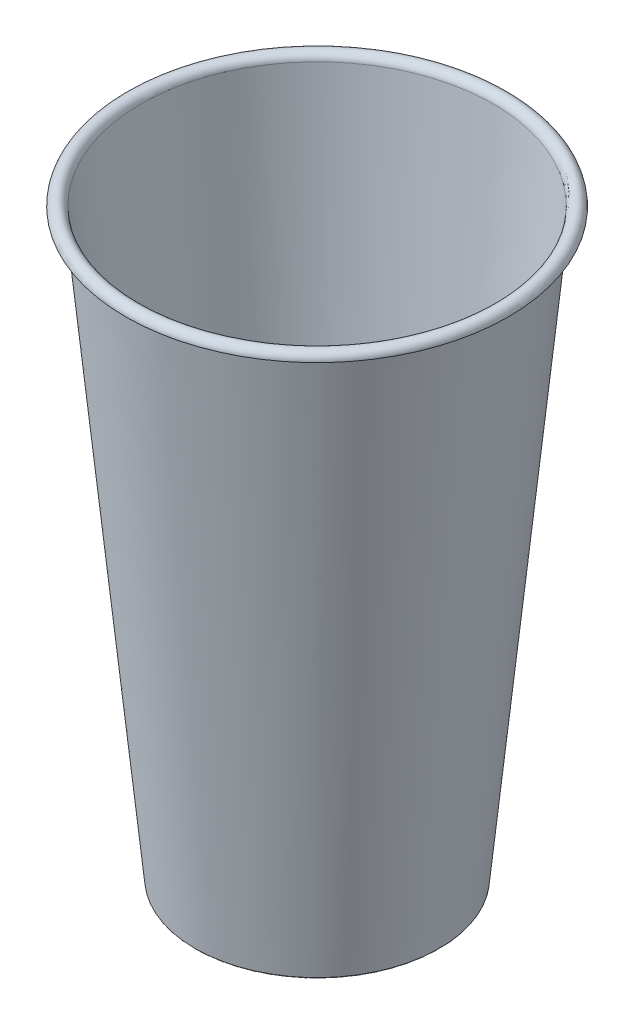
SolidWorks part; units mm, degrees
ref_plane "前视基准面" through (0, 0, 0) normal (0, 0, 1) x (1, 0, 0)
ref_plane "上视基准面" through (0, 0, 0) normal (0, 1, 0) x (1, 0, 0)
ref_plane "右视基准面" through (0, 0, 0) normal (1, 0, 0) x (0, 0, -1)
sketch "草图1" plane through (0, 0, 0) normal (0, 0, 1) x (1, 0, 0)
  line L0 (0, 0) -> (28.15, 0)
  line L1 (27.775, -3.8406) -> (28.0914, -0.6)
  line L2 (0, -0.6) -> (28.0914, -0.6)
  line L3 (28.374, -3.8794) -> (41.5972, 131.5417)
  line L4 (0, 0) -> (0, -0.6)
  line L5 (28.6943, -0.6) -> (41.5972, 131.5417) construction
  line L6 (27.974, -4.06) -> (28.175, -4.06)
  line L7 (28.15, 0) -> (41, 131.6) construction
  line L8 (0, -4.06) -> (28.6943, -4.06) construction
  line L9 (28.15, 0) -> (41, 131.6)
  line L10 (43.8917, 131.4299) -> (44.4917, 131.4299)
  line L11 (0, -0.6) -> (28.6943, -0.6) construction
  arc A0 (44.4917, 131.4299) -> (41, 131.6) centre (42.7417, 131.4299) ccw
  arc A1 (27.974, -4.06) -> (27.775, -3.8406) centre (27.974, -3.86) cw
  arc A2 (28.374, -3.8794) -> (28.175, -4.06) centre (28.175, -3.86) cw
  arc A3 (43.8917, 131.4299) -> (41.5972, 131.5417) centre (42.7417, 131.4299) ccw
  arc A5 (41.4992, 130.1976) -> (41, 131.6) centre (42.7417, 131.4299) ccw construction
  arc A6 (41.9252, 130.6201) -> (41.5972, 131.5417) centre (42.7417, 131.4299) ccw construction
  dimension "D6" = 0.2
  dimension "D7" = 1.75
  dimension "D1" = 28.15
  dimension "D2" = 131.6
  dimension "D3" = 41
  dimension "D4" = 0.6
  dimension "D5" = 3.46
revolve "旋转1" add sketch "草图1" angle 360 about L4
